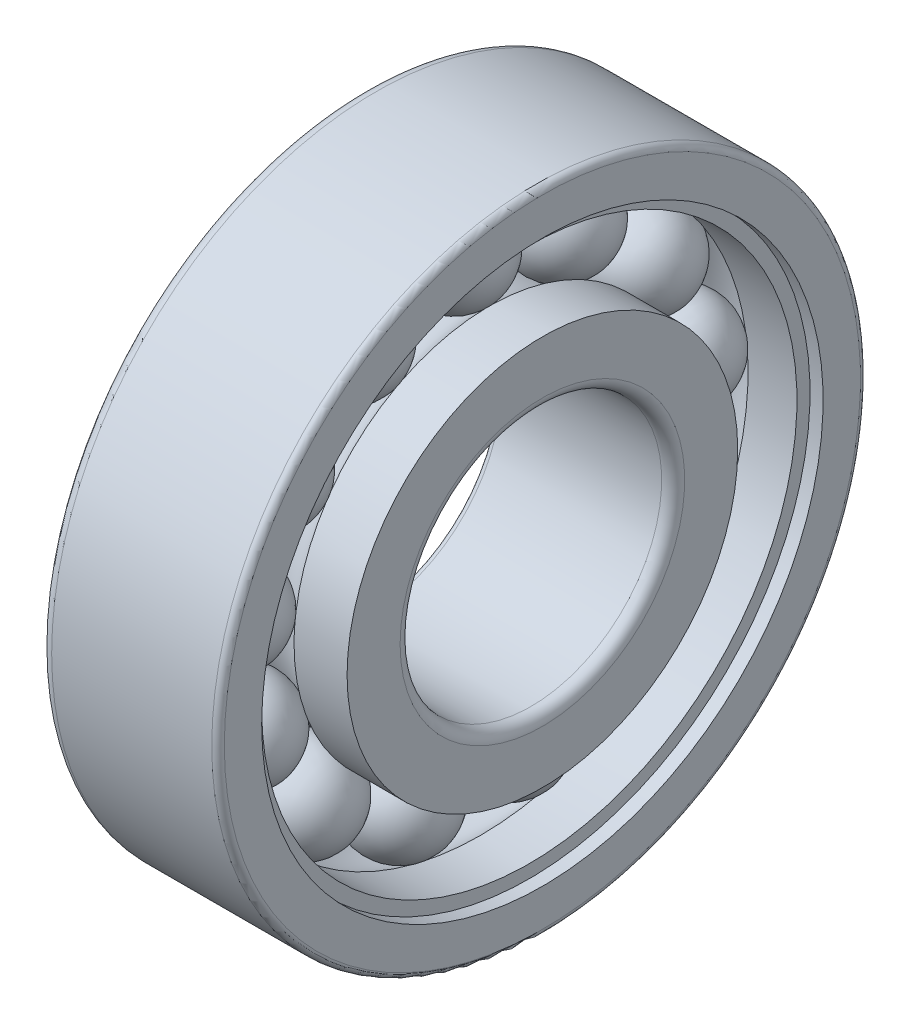
SolidWorks part; units mm, degrees
ref_plane "Front" through (0, 0, 0) normal (0, 0, 1) x (1, 0, 0)
ref_plane "Top" through (0, 0, 0) normal (0, 1, 0) x (1, 0, 0)
ref_plane "Right" through (0, 0, 0) normal (1, 0, 0) x (0, 0, -1)
sketch "Sketch1" plane through (0, 0, 0) normal (0, 0, 1) x (1, 0, 0)
  line L0 (-3.0919, 0) -> (2.899, 0) construction
  line L1 (-3.0919, 21.75) -> (2.899, 21.75) construction
  line L2 (-4.625, 21.75) -> (4.625, 21.75)
  arc A0 (-4.625, 21.75) -> (4.625, 21.75) centre (0, 21.75) ccw
revolve "Revolve1" add sketch "Sketch1" angle 360 about L1
sketch "Sketch2" plane through (0, 0, 0) normal (0, 0, 1) x (1, 0, 0)
  line L0 (-8.5, 18.6667) -> (-3.4338, 18.6667)
  line L1 (8.5, 18.6667) -> (8.5, 12.5)
  line L2 (8.5, 12.5) -> (-8.5, 12.5)
  line L3 (-8.5, 12.5) -> (-8.5, 18.6667)
  line L4 (-2.9924, 0) -> (3.9982, 0) construction
  line L5 (-1.8743, 21.75) -> (3.1755, 21.75) construction
  line L7 (3.4338, 18.6667) -> (8.5, 18.6667)
  line L8 (-8.5, 6.2861) -> (-8.5, 1.454) construction
  arc A0 (-3.4338, 18.6667) -> (3.4338, 18.6667) centre (0, 21.75) ccw
revolve "Revolve2" add sketch "Sketch2" angle 360 about L4
sketch "Sketch3" plane through (0, 0, 0) normal (0, 0, 1) x (1, 0, 0)
  line L0 (-8.5, 24.8333) -> (-8.5, 31)
  line L1 (-8.5, 31) -> (8.5, 31)
  line L2 (8.5, 31) -> (8.5, 26.8283)
  line L3 (7.25, 25.5783) -> (2.5772, 25.5783)
  line L4 (-2.9924, 0) -> (3.4329, 0) construction
  line L6 (-1.7375, 21.75) -> (2.2712, 21.75) construction
  line L7 (-3.4338, 24.8333) -> (-8.5, 24.8333)
  line L8 (7.25, 25.5783) -> (7.25, 26.8283)
  line L9 (7.25, 26.8283) -> (8.5, 26.8283)
  arc A0 (2.5772, 25.5783) -> (-3.4338, 24.8333) centre (0, 21.75) ccw
revolve "Revolve3" add sketch "Sketch3" angle 360 about L4
pattern_circular "Circular-Pattern1" count 13 over 360 about axis through (0, 0, 0) along (1, 0, 0) of "Revolve1"
fillet "Fillet1" radius 1.1 2 edges at (8.5, 0, 12.5) (-8.5, 0, 31)
fillet "Fillet2" radius 0.6 2 edges at (8.5, 0, 31) (-8.5, 0, 12.5)
equation "\"R@Sketch1\" =  ( \"DD@Sketch3\" - \"d@Sketch2\" )  / 8"
equation "\"D1@Sketch1\"=(\"d@Sketch2\"+\"DD@Sketch3\")/4"
equation "\"D1@Sketch2\"=(\"d@Sketch2\"+\"DD@Sketch3\")/4"
equation "\"D3@Sketch2\" =  \"d@Sketch2\"+  ( \"DD@Sketch3\" - \"d@Sketch2\" )  /3"
equation "\"D2@Sketch2\" =  ( \"DD@Sketch3\" - \"d@Sketch2\" )  / 8 - 0.01"
equation "\"D6@Sketch2\" = \"B@Sketch2\" / 2"
equation "\"B@Sketch3\" = \"B@Sketch2\""
equation "\"D2@Sketch3\" = \"B@Sketch3\" / 2"
equation "\"D1@Sketch3\"=(\"d@Sketch2\"+\"DD@Sketch3\")/4"
equation "\"D3@Sketch3\" = (  \"DD@Sketch3\" -  (\"DD@Sketch3\" - \"d@Sketch2\"  )  / 3 )  * 1.03"
equation "\"D5@Sketch3\" = \"DD@Sketch3\" -  (  \"DD@Sketch3\" - \"d@Sketch2\")  / 3"
equation "\"D6@Sketch3\" = \"d@Sketch2\" / 20"
equation "\"D7@Sketch3\"=\"D6@Sketch3\""
equation "\"D4@Sketch3\"=(\"DD@Sketch3\"-\"d@Sketch2\")/8-0.01"
equation "\"m@Circular-Pattern1\" = int( 3.14159265 / atn(\"R@Sketch1\" / sqr((\"d@Sketch2\"+\"DD@Sketch3\")/4 * (\"d@Sketch2\"+\"DD@Sketch3\")/4 - \"R@Sketch1\" *  \"R@Sketch1\")))-1"
